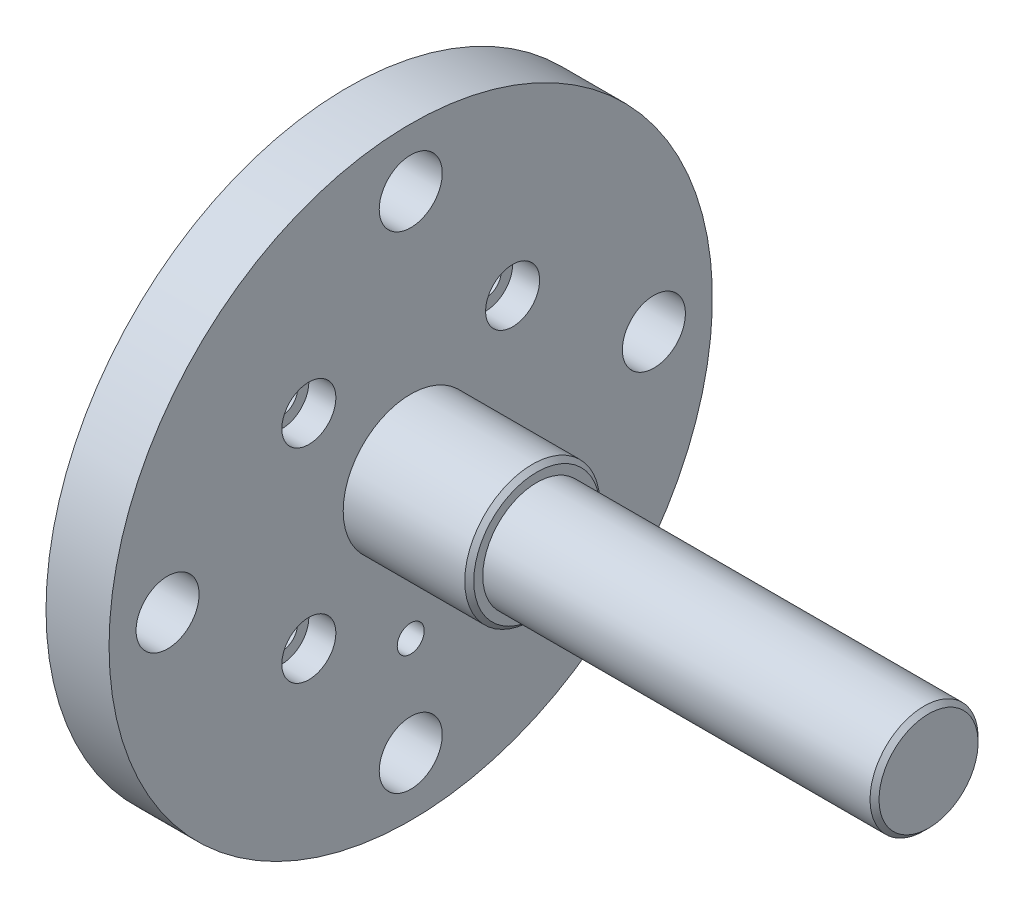
SolidWorks part; units mm, degrees
material "S45C"
ref_plane "Front Plane" through (0, 0, 0) normal (0, 0, 1) x (1, 0, 0)
ref_plane "Top Plane" through (0, 0, 0) normal (0, 1, 0) x (1, 0, 0)
ref_plane "Right Plane" through (0, 0, 0) normal (1, 0, 0) x (0, 0, -1)
sketch "Sketch1" plane through (0, 0, 0) normal (0, 0, 1) x (1, 0, 0)
  line L0 (0, 0) -> (142.1888, 0) construction
  line L1 (0, 0) -> (0, 8)
  line L2 (0, 8) -> (75, 8)
  line L3 (75, 8) -> (75, 17.5)
  line L4 (75, 17.5) -> (82, 17.5)
  line L5 (82, 17.5) -> (82, 34)
  line L6 (82, 34) -> (92, 34)
  line L7 (92, 34) -> (92, 15)
  line L8 (92, 15) -> (120, 15)
  line L9 (120, 15) -> (120, 12)
  line L10 (120, 12) -> (207, 12)
  line L11 (207, 12) -> (207, 0)
  line L12 (207, 0) -> (0, 0)
  dimension "D1" = 16
  dimension "D2" = 17.5
  dimension "D3" = 34
  dimension "D4" = 15
  dimension "D5" = 12
  dimension "D6" = 75
  dimension "D7" = 7
  dimension "D8" = 10
  dimension "D9" = 28
  dimension "D10" = 87
revolve "Revolve1" add sketch "Sketch1" angle 360 about L0
sketch "Sketch2" plane through (92, 0, 0) normal (1, 0, 0) x (0, 0, -1)
  circle A0 centre (0, 24.5) radius 3.5
  dimension "D2" = 7
  dimension "D1" = 24.5
extrude "Cut-Extrude1" cut sketch "Sketch2" against normal blind 27
sketch "Sketch3" plane through (82, 0, 0) normal (-1, 0, 0) x (0, 0, 1)
  circle A0 centre (0, 24.5) radius 5.5
  dimension "D1" = 11
extrude "Cut-Extrude2" cut sketch "Sketch3" against normal blind 6
pattern_circular "CirPattern1" count 4 over 360 about axis through (0, 0, 0) along (1, 0, 0) of "Cut-Extrude2", "Cut-Extrude1"
chamfer "Chamfer1" distance 1 angle 45 6 edges at (207, 0, 12) (75, 0, 17.5) (75, 0, 8) (0, 0, 8) (120, 0, 15) (82, 0, 34)
sketch "Sketch4" plane through (92, 0, 0) normal (1, 0, 0) x (0, 0, -1)
  circle A0 centre (0, 0) radius 52.9106
extrude "Cut-Extrude3" cut sketch "Sketch4" against normal blind 128
sketch "Sketch5" plane through (92, 0, 0) normal (-1, 0, 0) x (0, 0, 1)
  circle A0 centre (0, 0) radius 67
  dimension "D1" = 134
extrude "Boss-Extrude1" add sketch "Sketch5" along normal blind 14
sketch "Sketch6" plane through (78, 0, 0) normal (-1, 0, 0) x (0, 0, 1)
  circle A0 centre (0, 0) radius 19
  dimension "D1" = 38
extrude "Boss-Extrude2" add sketch "Sketch6" along normal blind 5
sketch "Sketch7" plane through (78, 0, 0) normal (-1, 0, 0) x (0, 0, 1)
  line L0 (0, 0) -> (22.6274, 22.6274) construction
  line L1 (0, 0) -> (0, 32) construction
  circle A0 centre (0, 0) radius 32 construction
  circle A1 centre (0, -32) radius 3
  circle A2 centre (22.6274, 22.6274) radius 3.5
  circle A3 centre (22.6274, -22.6274) radius 3.5
  circle A4 centre (-22.6274, -22.6274) radius 3.5
  circle A5 centre (-22.6274, 22.6274) radius 3.5
  dimension "D1" = 64
  dimension "D2" = 6
  dimension "D4" = 7
  dimension "D3" = 45
  dimension "D5" = 4
extrude "Cut-Extrude4" cut sketch "Sketch7" against normal blind 41
sketch "Sketch8" plane through (92, 0, 0) normal (1, 0, 0) x (0, 0, -1)
  circle A0 centre (22.6274, 22.6274) radius 6
  circle A1 centre (22.6274, -22.6274) radius 6
  circle A2 centre (-22.6274, -22.6274) radius 6
  circle A3 centre (-22.6274, 22.6274) radius 6
  dimension "D1" = 12
extrude "Cut-Extrude5" cut sketch "Sketch8" against normal blind 6
chamfer "Chamfer2" distance 1 angle 45 1 edges at (73, 0, 19)
sketch "Sketch9" plane through (78, 0, 0) normal (-1, 0, 0) x (0, 0, 1)
  circle A0 centre (0, -54) radius 7
  dimension "D2" = 14
  dimension "D1" = 54
extrude "Cut-Extrude6" cut sketch "Sketch9" against normal blind 41
pattern_circular "CirPattern2" count 4 over 360 about axis through (0, 0, 0) along (1, 0, 0) of "Cut-Extrude6"
